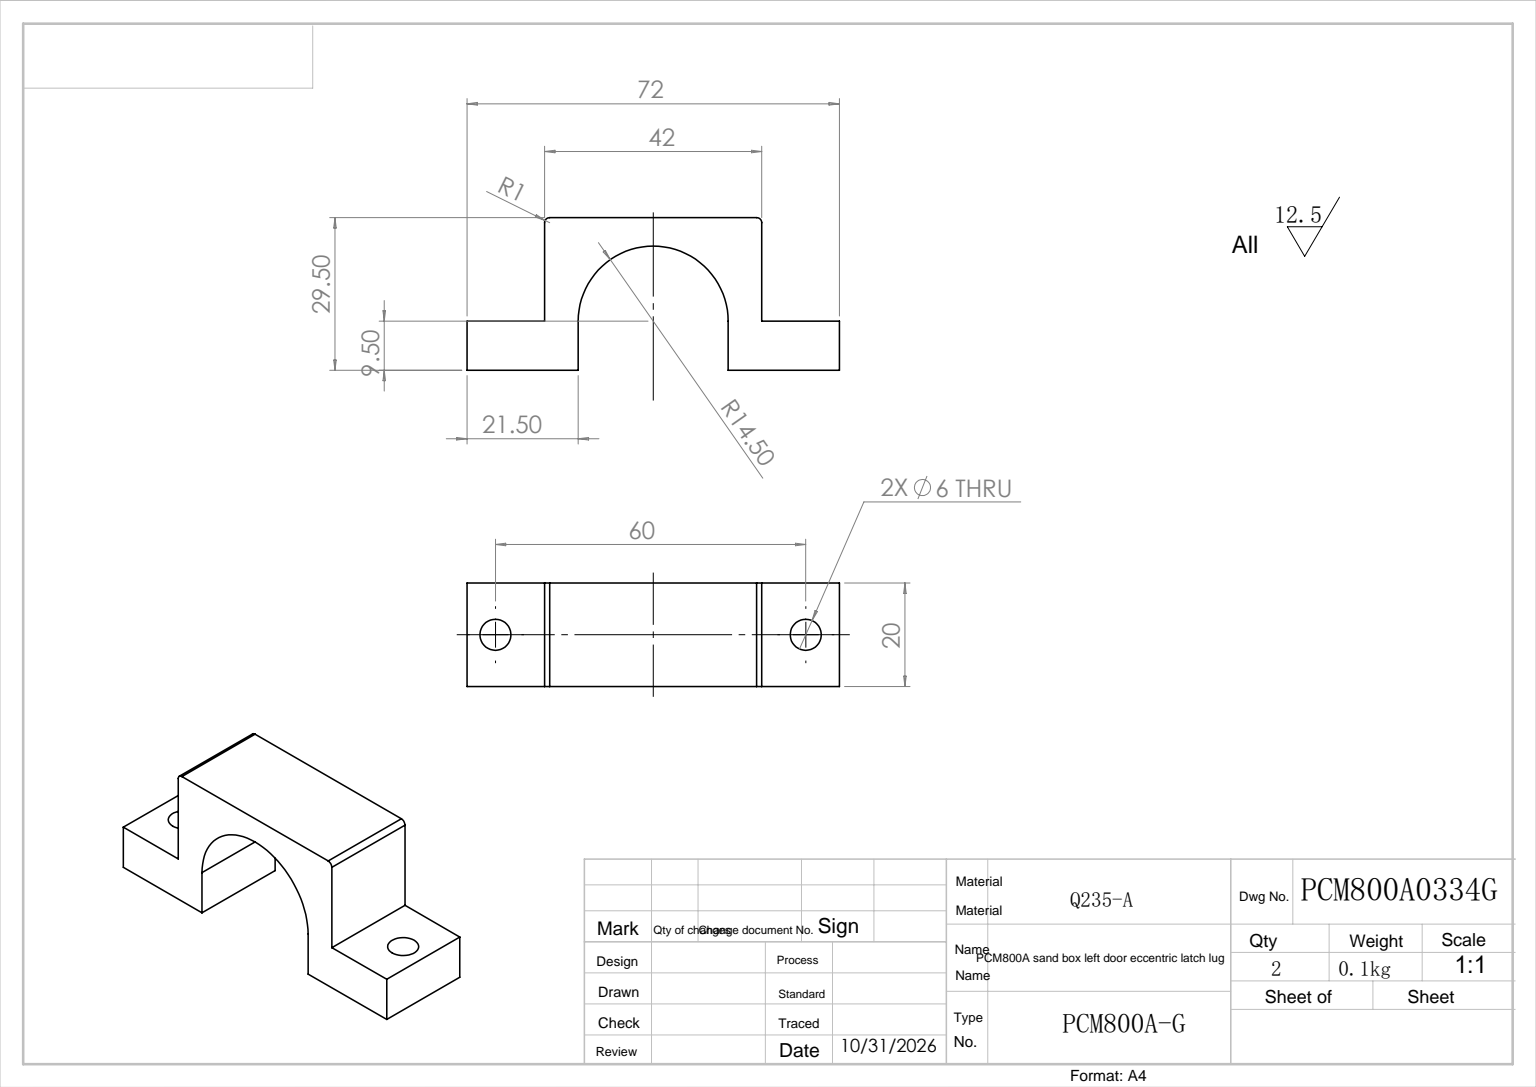
SolidWorks part; units mm, degrees
ref_plane "前视基准面" through (0, 0, 0) normal (0, 0, 1) x (1, 0, 0)
ref_plane "上视基准面" through (0, 0, 0) normal (0, 1, 0) x (1, 0, 0)
ref_plane "右视基准面" through (0, 0, 0) normal (1, 0, 0) x (0, 0, -1)
sketch "草图1" plane through (0, 0, 0) normal (0, 0, 1) x (1, 0, 0)
  line L0 (0, 0) -> (15, 0)
  line L1 (15, 0) -> (15, 20)
  line L2 (15, 20) -> (57, 20)
  line L3 (57, 20) -> (57, 0)
  line L4 (57, 0) -> (72, 0)
  line L5 (72, 0) -> (72, -9.5)
  line L6 (21.5, 0) -> (21.5, -9.5)
  line L7 (50.5, 0) -> (50.5, -9.5)
  line L8 (21.5, -9.5) -> (0, -9.5)
  line L10 (72, -9.5) -> (50.5, -9.5)
  line L11 (0, -9.5) -> (0, 0)
  arc A0 (50.5, 0) -> (21.5, 0) centre (36, 0) ccw
  dimension "D6" = 29
  dimension "D7" = 9.5
  dimension "D8" = 36
  dimension "D1" = 42
  dimension "D2" = 15
  dimension "D3" = 15
  dimension "D4" = 29.5
  dimension "D5" = 9.5
extrude "凸台-拉伸1" add sketch "草图1" along normal blind 20
fillet "圆角1" radius 1 2 edges at (57, 20, 10) (15, 20, 10)
sketch "草图2" plane through (0, 0, 0) normal (0, 1, 0) x (1, 0, 0)
  line L0 (72, -20) -> (72, 0) construction
  circle A0 centre (6.5, -10) radius 3
  circle A1 centre (66.5, -10) radius 3
  dimension "D1" = 6
  dimension "D2" = 5.5
  dimension "D3" = 60
extrude "切除-拉伸1" cut sketch "草图2" against normal through all
